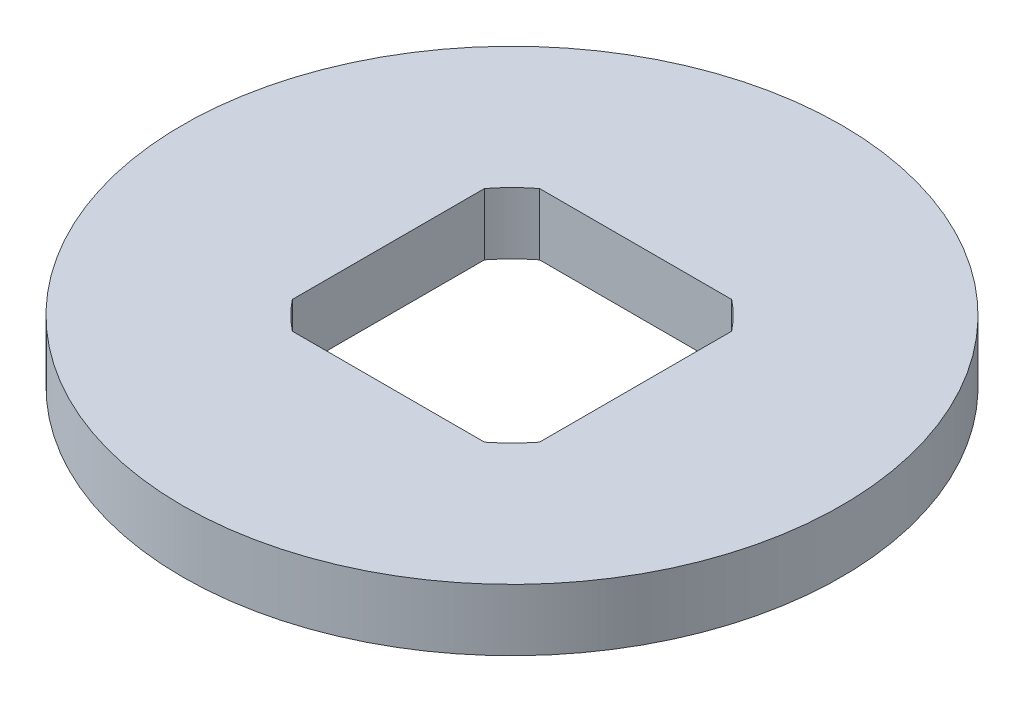
SolidWorks part; units mm, degrees
ref_plane "Front Plane" through (0, 0, 0) normal (0, 0, 1) x (1, 0, 0)
ref_plane "Top Plane" through (0, 0, 0) normal (0, 1, 0) x (1, 0, 0)
ref_plane "Right Plane" through (0, 0, 0) normal (1, 0, 0) x (0, 0, -1)
ref_plane "Plane4" through (0, -1.5, 0) normal (0, -1, 0) x (1, 0, 0)
sketch "Sketch1" plane through (0, -1.5, 0) normal (0, -1, 0) x (1, 0, 0)
  line L0 (3, 2.3324) -> (3, -2.3324)
  line L1 (2.3324, -3) -> (-2.3324, -3)
  line L2 (-3, -2.3324) -> (-3, 2.3324)
  line L3 (-2.3324, 3) -> (2.3324, 3)
  arc A0 (2.3324, 3) -> (3, 2.3324) centre (0, 0) cw
  arc A1 (3, -2.3324) -> (2.3324, -3) centre (0, 0) cw
  arc A2 (-2.3324, -3) -> (-3, -2.3324) centre (0, 0) cw
  arc A3 (-3, 2.3324) -> (-2.3324, 3) centre (0, 0) cw
  circle A4 centre (0, 0) radius 8
extrude "Boss-Extrude1" add sketch "Sketch1" against normal blind 1.5
